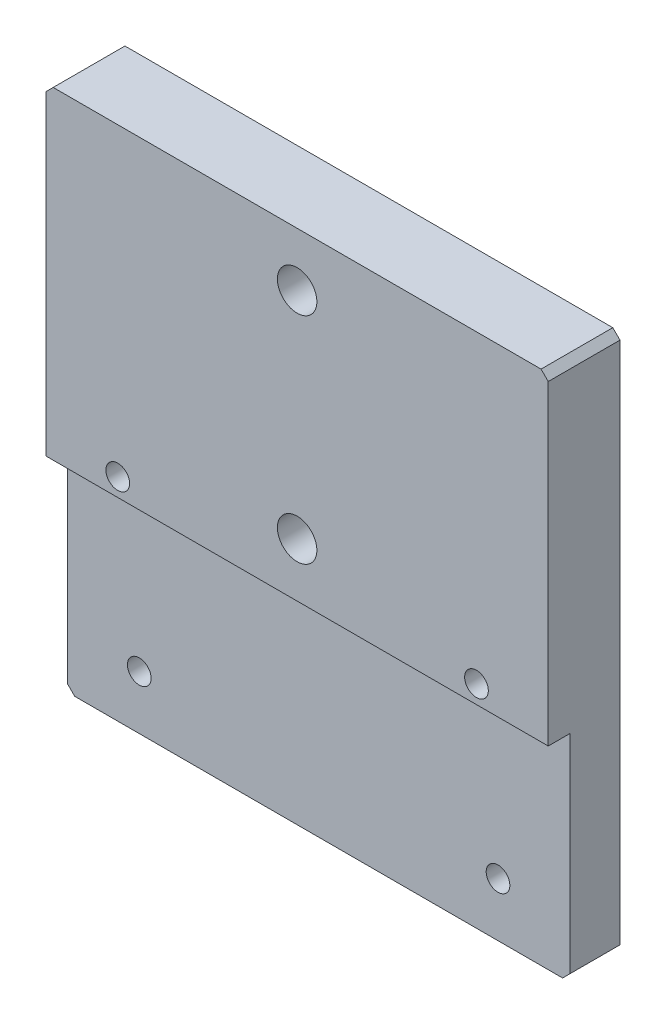
from build123d import *

# Parameters (mm, degrees)
SKETCH1_W                                            = 70
SKETCH1_H                                            = 75
BOSS_EXTRUDE1_DEPTH                                  = 10
SKETCH2_W                                            = 3
SKETCH2_H                                            = 30
CUT_EXTRUDE1_DEPTH                                   = 104.07764064
M4_TAPPED_HOLE1_D                                    = 3.3
M4_TAPPED_HOLE1_DEPTH                                = 11.5
M4_TAPPED_HOLE1_TIP                                  = 0.991420021
HOLE_SIZE_PER_SOCKET_HEAD_CAP_SCREW_TYPE_D           = 5.5
HOLE_SIZE_PER_SOCKET_HEAD_CAP_SCREW_TYPE_CBORE_D     = 10
HOLE_SIZE_PER_SOCKET_HEAD_CAP_SCREW_TYPE_CBORE_DEPTH = 5.7
CHAMFER1_SIZE                                        = 1


with BuildPart() as part:
    # Sketch1 → Boss-Extrude1 (new body)
    with BuildSketch(Plane.XY):
        with Locations((35, 37.5)):
            Rectangle(SKETCH1_W, SKETCH1_H)
    extrude(amount=BOSS_EXTRUDE1_DEPTH)

    # Sketch2 → Cut-Extrude1 (cut, through all)
    with BuildSketch(Plane.ZY):
        with Locations((8.5, 15)):
            Rectangle(SKETCH2_W, SKETCH2_H)
    extrude(amount=-CUT_EXTRUDE1_DEPTH, mode=Mode.SUBTRACT)

    # M4 Tapped Hole1
    with Locations(Plane(origin=(0, 0, 0), x_dir=(-1, 0, 0), z_dir=(0, 0, -1))):
        with Locations((-10, 7.5), (-10, 32.5), (-60, 7.5), (-60, 32.5)):
            Hole(M4_TAPPED_HOLE1_D / 2, depth=M4_TAPPED_HOLE1_DEPTH)
            with Locations((0, 0, -(M4_TAPPED_HOLE1_DEPTH + M4_TAPPED_HOLE1_TIP / 2))):  # 118° drill point
                Cone(0, M4_TAPPED_HOLE1_D / 2, M4_TAPPED_HOLE1_TIP, mode=Mode.SUBTRACT)

    # Hole Size per Socket Head Cap Screw Type0 (through all)
    with Locations(Plane(origin=(0, 0, 0), x_dir=(-1, 0, 0), z_dir=(0, 0, -1))):
        with Locations((-35, 37.5), (-35, 67.5)):
            CounterBoreHole(HOLE_SIZE_PER_SOCKET_HEAD_CAP_SCREW_TYPE_D / 2, HOLE_SIZE_PER_SOCKET_HEAD_CAP_SCREW_TYPE_CBORE_D / 2, HOLE_SIZE_PER_SOCKET_HEAD_CAP_SCREW_TYPE_CBORE_DEPTH)

    # Chamfer1
    chamfer1_edges = [part.edges().sort_by_distance(p)[0] for p in [
        (70, 0, 3.5),
        (0, 0, 3.5),
        (0, 75, 5),
        (70, 75, 5),
    ]]
    chamfer(chamfer1_edges, length=CHAMFER1_SIZE)


solid = part.part
